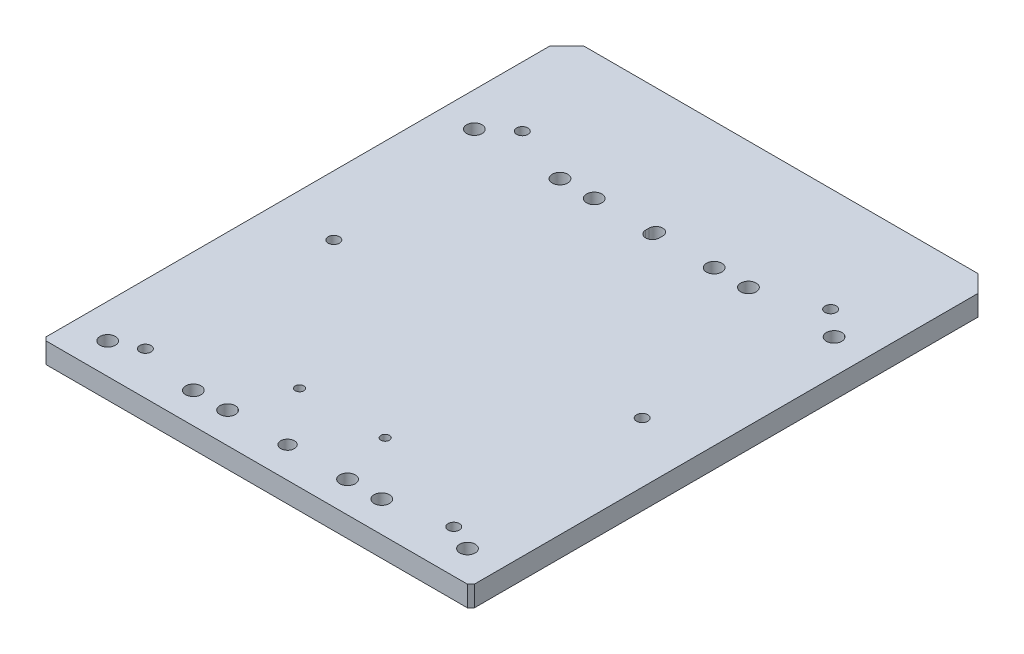
from build123d import *

# Parameters (mm, degrees)
SKETCH_1_W                = 250
SKETCH_1_H                = 306
EXTRUDE_1_DEPTH           = 6
CHAMFER_1_SIZE            = 2
HOLE_WIZARD_M6_1_D        = 5
HOLE_WIZARD_M6_1_DEPTH    = 15
HOLE_WIZARD_M6_1_TIP      = 1.502151548
HOLE_WIZARD_M8_1_D        = 9
HOLE_WIZARD_1_D           = 6.6
HOLE_WIZARD_1_CBORE_D     = 11
HOLE_WIZARD_1_CBORE_DEPTH = 6.8
SKETCH_8_R                = 4
CUT_EXTRUDE_1_DEPTH       = 198.934332545
HOLE_WIZARD_M6_2_D        = 5
CHAMFER_2_SIZE            = 10


with BuildPart() as part:
    # 草图1 → 凸台-拉伸1 (new, symmetric)
    with BuildSketch(Plane(origin=(0, 0, 0), x_dir=(1, 0, 0), z_dir=(0, 1, 0))):
        Rectangle(SKETCH_1_W, SKETCH_1_H)
    extrude(amount=EXTRUDE_1_DEPTH, both=True)

    # 倒角1
    chamfer_1_edges = [part.edges().sort_by_distance(p)[0] for p in [
        (125, 0, 153),
        (-125, 0, 153),
    ]]
    chamfer(chamfer_1_edges, length=CHAMFER_1_SIZE)

    # M6 螺纹孔1
    with Locations(Plane(origin=(0, 0, -153), x_dir=(-1, 0, 0), z_dir=(0, 0, -1))):
        with Locations((-105, 0), (0, 0), (105, 0)):
            Hole(HOLE_WIZARD_M6_1_D / 2, depth=HOLE_WIZARD_M6_1_DEPTH)
            with Locations((0, 0, -(HOLE_WIZARD_M6_1_DEPTH + HOLE_WIZARD_M6_1_TIP / 2))):  # 118° drill point
                Cone(0, HOLE_WIZARD_M6_1_D / 2, HOLE_WIZARD_M6_1_TIP, mode=Mode.SUBTRACT)

    # M8 间隙孔1 (through all)
    with Locations(Plane(origin=(0, 6, 0), x_dir=(1, 0, 0), z_dir=(0, 1, 0))):
        with Locations((-105, -135.00000089), (-55, -135.00000089), (-105, 78.99999911), (-55, 78.99999911), (55, 78.99999911), (105, 78.99999911), (55, -135.00000089), (105, -135.00000089), (-35, -135.00000089), (35, -135.00000089), (-35, 78.99999911), (35, 78.99999911)):
            Hole(HOLE_WIZARD_M8_1_D / 2)

    # 打孔尺寸(%根据)内六角圆柱头螺钉的类型1 (through all)
    with Locations(Plane(origin=(0, -6, 0), x_dir=(-1, 0, 0), z_dir=(0, -1, 0))):
        with Locations((-90, -128), (-90, -18), (-90, 92), (90, 92), (90, -18), (90, -128)):
            CounterBoreHole(HOLE_WIZARD_1_D / 2, HOLE_WIZARD_1_CBORE_D / 2, HOLE_WIZARD_1_CBORE_DEPTH)

    # 草图8 → 切除-拉伸1 (cut, through all)
    with BuildSketch(Plane(origin=(0, 6, 0), x_dir=(1, 0, 0), z_dir=(0, 1, 0))):
        with Locations(Location((0, -135.00000089, 0), (0, 0, 270))):
            Circle(SKETCH_8_R)
        with BuildLine():
            Line((-4, 77.99999911), (-4, 79.99999911))
            ThreePointArc((-4, 79.99999911), (0, 83.99999911), (4, 79.99999911))
            Line((4, 79.99999911), (4, 77.99999911))
            ThreePointArc((4, 77.99999911), (0, 73.99999911), (-4, 77.99999911))
        make_face()
    extrude(amount=-CUT_EXTRUDE_1_DEPTH, mode=Mode.SUBTRACT)

    # M6 螺纹孔2 (through all)
    with Locations(Plane(origin=(0, 6, 0), x_dir=(1, 0, 0), z_dir=(0, 1, 0))):
        with Locations((25, -103), (-25, -103)):
            Hole(HOLE_WIZARD_M6_2_D / 2)

    # 倒角2
    chamfer_2_edges = [part.edges().sort_by_distance(p)[0] for p in [
        (-125, 0, -153),
        (125, 0, -153),
    ]]
    chamfer(chamfer_2_edges, length=CHAMFER_2_SIZE)


solid = part.part
